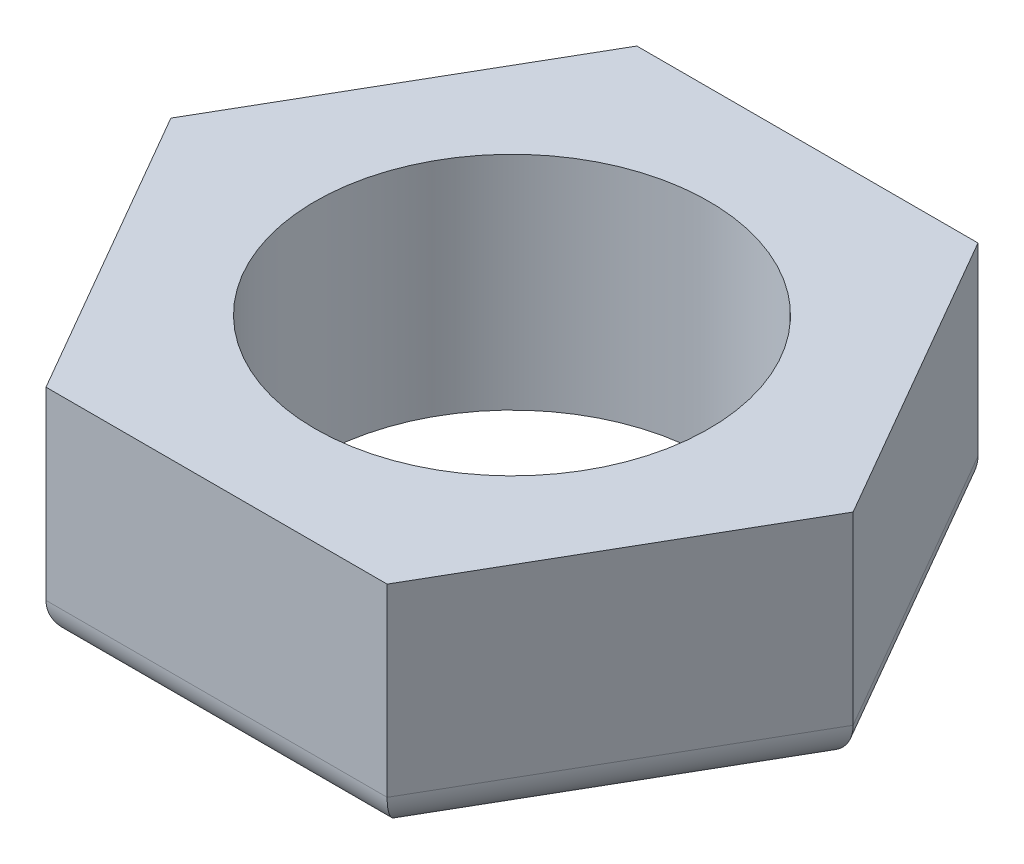
SolidWorks part; units mm, degrees
ref_plane "Front Plane" through (0, 0, 0) normal (0, 0, 1) x (1, 0, 0)
ref_plane "Top Plane" through (0, 0, 0) normal (0, 1, 0) x (1, 0, 0)
ref_plane "Right Plane" through (0, 0, 0) normal (1, 0, 0) x (0, 0, -1)
sketch "Sketch1" plane through (0, 0, 0) normal (0, 1, 0) x (1, 0, 0)
  line L1 (13.8564, 0) -> (6.9282, 12)
  line L2 (6.9282, 12) -> (-6.9282, 12)
  line L3 (-6.9282, 12) -> (-13.8564, 0)
  line L4 (-13.8564, 0) -> (-6.9282, -12)
  line L5 (-6.9282, -12) -> (6.9282, -12)
  line L6 (6.9282, -12) -> (13.8564, 0)
  circle A1 centre (0, 0) radius 8
  dimension "D1" = 24
extrude "Extrude1" add sketch "Sketch1" along normal blind 9
fillet "Fillet1" radius 1.5 6 edges at (10.3923, 0, -6) (10.3923, 0, 6) (0, 0, 12) (-10.3923, 0, 6) (-10.3923, 0, -6) (0, 0, -12)
